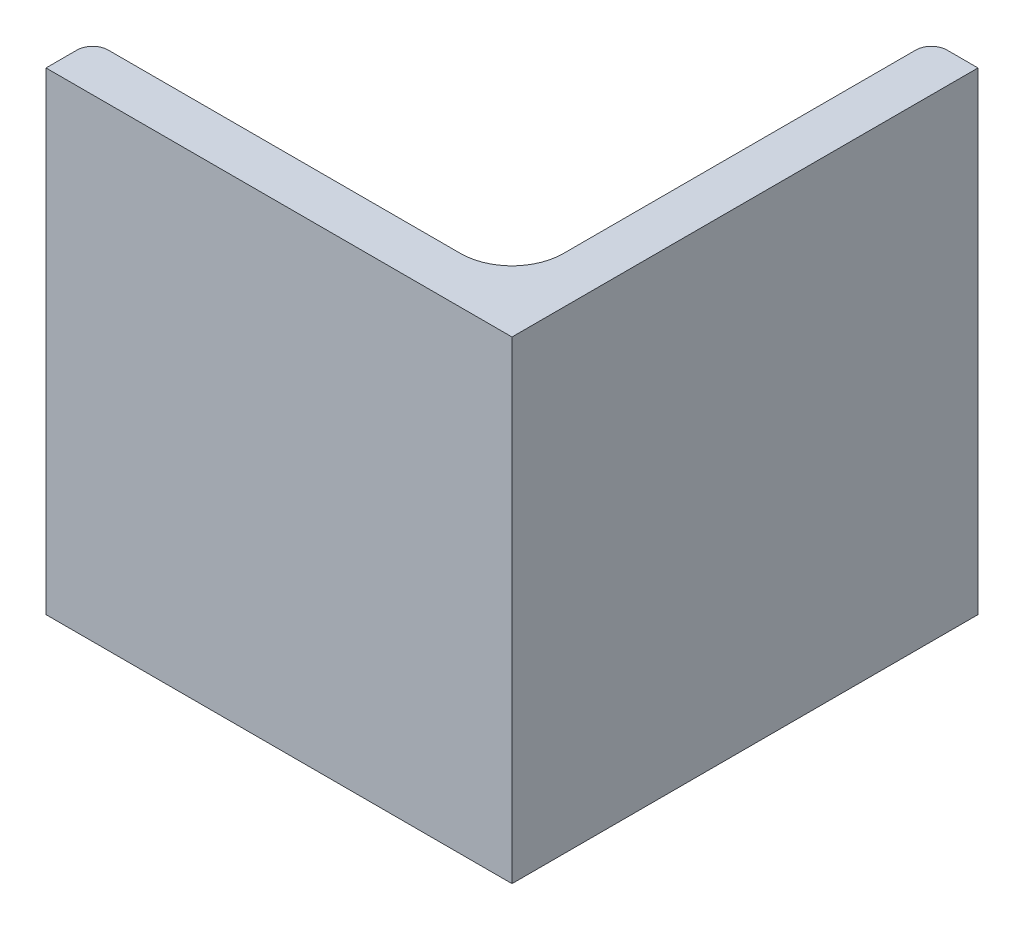
SolidWorks part; units mm, degrees
material "Q235B"
ref_plane "Front Plane" through (0, 0, 0) normal (0, 0, 1) x (1, 0, 0)
ref_plane "Top Plane" through (0, 0, 0) normal (0, 1, 0) x (1, 0, 0)
ref_plane "Right Plane" through (0, 0, 0) normal (1, 0, 0) x (0, 0, -1)
sketch "Sketch1" plane through (0, 0, 0) normal (0, 1, 0) x (1, 0, 0)
  line L0 (-163.5028, 0) -> (105.3138, 0) construction
  line L1 (0, 168.0104) -> (0, -160.6343) construction
  line L2 (0, -25) -> (0, 25)
  line L3 (0, 25) -> (-5, 25)
  line L4 (-5, 25) -> (-5, -20)
  line L5 (-5, -20) -> (-50, -20)
  line L6 (-50, -20) -> (-50, -25)
  line L7 (-50, -25) -> (0, -25)
  point P5 (-25, -25)
  point P8 (0, 0)
  dimension "D1" = 50
  dimension "D2" = 5
  dimension "D3" = 50
extrude "Extrude1" add sketch "Sketch1" along normal mid plane 50.8
fillet "Fillet1" radius 5.5 1 edges at (-5, 0, 20)
fillet "Fillet2" radius 1.67 2 edges at (-50, 0, 20) (-5, 0, -25)
